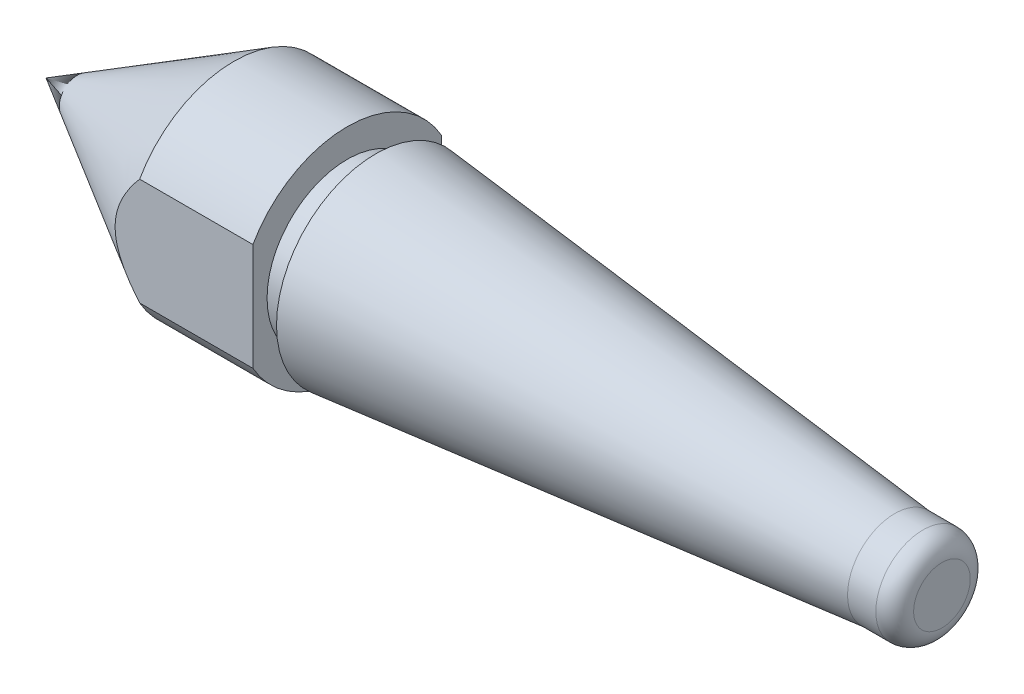
SolidWorks part; units mm, degrees
ref_plane "Front Plane" through (0, 0, 0) normal (0, 0, 1) x (1, 0, 0)
ref_plane "Top Plane" through (0, 0, 0) normal (0, 1, 0) x (1, 0, 0)
ref_plane "Right Plane" through (0, 0, 0) normal (1, 0, 0) x (0, 0, -1)
other "Configuration Table"
sketch "Sketch1" plane through (0, 0, 0) normal (0, 0, 1) x (1, 0, 0)
  line L0 (0, 0) -> (-110.6848, 0) construction
  line L1 (0, 0) -> (0, 5)
  line L2 (0, 5) -> (-5, 5)
  line L3 (-5, 5) -> (-60, 10.5)
  line L4 (-60, 10.5) -> (-60, 8.5)
  line L5 (-60, 8.5) -> (-63, 8.5)
  line L6 (-63, 8.5) -> (-63, 11.5)
  line L8 (-94.92, 0) -> (0, 0)
  line L9 (-63, 11.5) -> (-75, 11.5)
  line L10 (-75, 11.5) -> (-94.92, 0)
  line L11 (-5, 5) -> (-8, 5) construction
  line L12 (-8, 5) -> (-8, 5.3) construction
  point P11 (-61.5, 8.5)
  dimension "D1" = 94.92
  dimension "D2" = 17
  dimension "D3" = 23
  dimension "D4" = 5
  dimension "D5" = 3
  dimension "D6" = 12
  dimension "D7" = 5
  dimension "D8" = 63
  dimension "D9" = 3
  dimension "D10" = 0.3
revolve "Revolve1" add sketch "Sketch1" angle 360 about L8
fillet "Fillet1" radius 2 1 edges at (0, 0, 5)
sketch "Sketch2" plane through (-63, 0, 0) normal (1, 0, 0) x (0, 0, -1)
  line L0 (7.158, 9.0007) -> (10, 12.5742) construction
  line L2 (-10, 5.6789) -> (-10, -5.6789)
  line L4 (10, 5.6789) -> (10, -5.6789)
  line L5 (-10, 12.5742) -> (-7.158, 9.0007) construction
  line L6 (-10, -12.5742) -> (0, 0) construction
  arc A0 (-10, 5.6789) -> (-10, -5.6789) centre (0, 0) ccw
  arc A1 (10, -5.6789) -> (10, 5.6789) centre (0, 0) ccw
  dimension "D1" = 23
extrude "Cut-Extrude1" cut sketch "Sketch2" against normal through all
